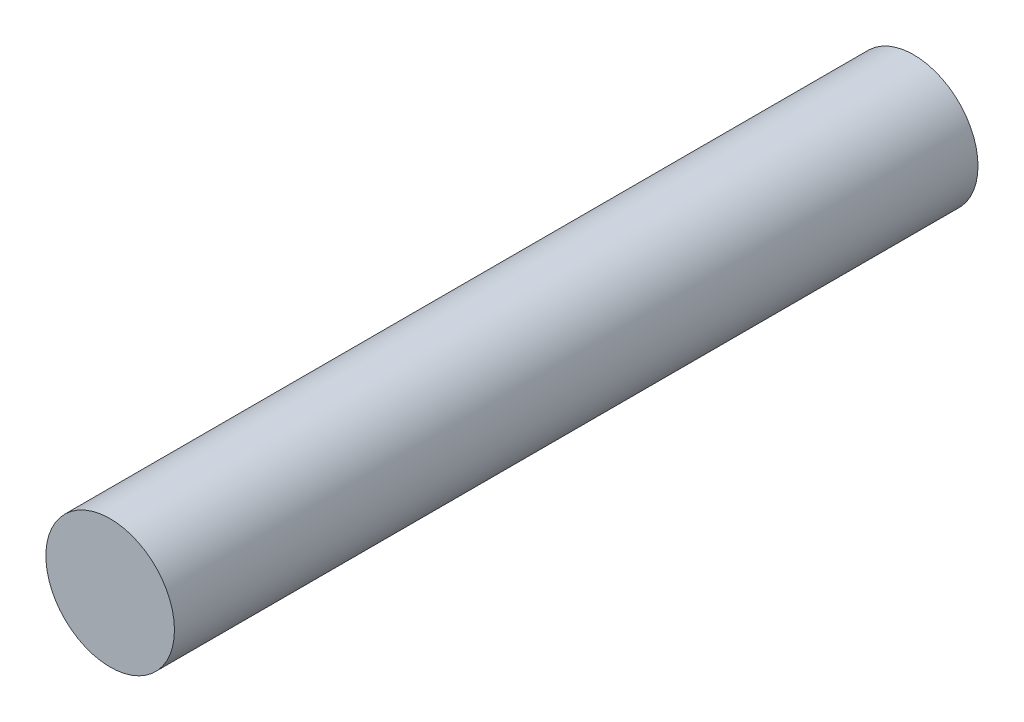
SolidWorks part; units mm, degrees
ref_plane "前视基准面" through (0, 0, 0) normal (0, 0, 1) x (1, 0, 0)
ref_plane "上视基准面" through (0, 0, 0) normal (0, 1, 0) x (1, 0, 0)
ref_plane "右视基准面" through (0, 0, 0) normal (1, 0, 0) x (0, 0, -1)
sketch "草图1" plane through (0, 0, 0) normal (0, 0, 1) x (1, 0, 0)
  circle A0 centre (0, 0) radius 6
  dimension "D1" = 12
extrude "凸台-拉伸1" add sketch "草图1" along normal mid plane 75
